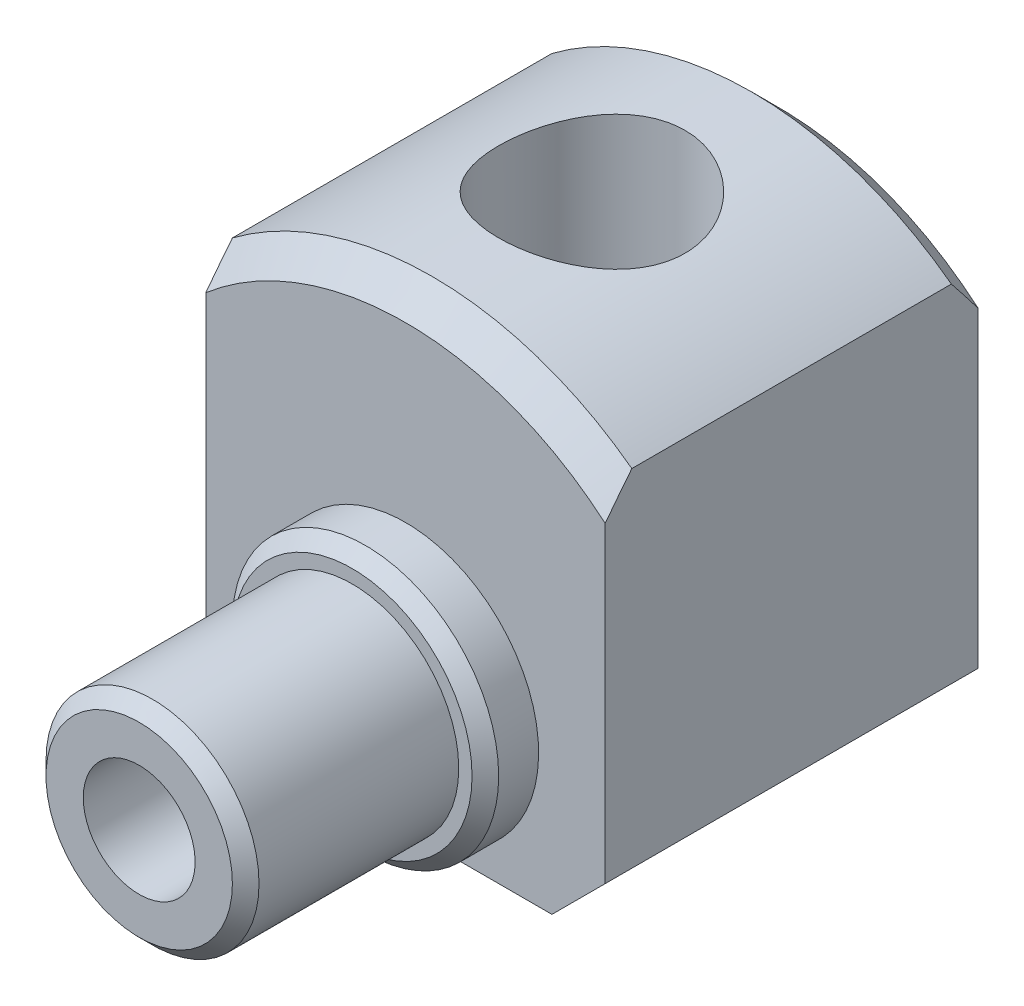
SolidWorks part; units mm, degrees
material "SUS304"
ref_plane "Front Plane" through (0, 0, 0) normal (0, 0, 1) x (1, 0, 0)
ref_plane "Top Plane" through (0, 0, 0) normal (0, 1, 0) x (1, 0, 0)
ref_plane "Right Plane" through (0, 0, 0) normal (1, 0, 0) x (0, 0, -1)
sketch "Sketch1" plane through (0, 0, 0) normal (0, 0, 1) x (1, 0, 0)
  circle A0 centre (0, 0) radius 12.5
  dimension "D1" = 25
extrude "Boss-Extrude1" add sketch "Sketch1" along normal mid plane 24
sketch "Sketch2" plane through (0, 0, 12) normal (0, 0, 1) x (1, 0, 0)
  circle A0 centre (0, 0) radius 4
  dimension "D1" = 8
extrude "Cut-Extrude1" cut sketch "Sketch2" against normal blind 10 flip side to cut
sketch "Sketch9" plane through (0, 0, -12) normal (0, 0, -1) x (-1, 0, 0)
  line L0 (0, 0) -> (0, 28.2403) construction
  line L1 (-7.5, 15) -> (7.5, 15)
  line L2 (-7.5, 15) -> (-7.5, -5)
  line L3 (-7.5, -5) -> (7.5, -5)
  line L4 (7.5, 15) -> (7.5, -5)
  dimension "D1" = 5
  dimension "D2" = 15
  dimension "D3" = 20
extrude "Cut-Extrude2" cut sketch "Sketch9" against normal through all flip side to cut
hole_wizard "M5 Tapped Hole1" positions "Sketch4" profile "Sketch3" tap size "M5" standard "GB" end condition through all
sketch "Sketch4" plane through (0, 0, -12) normal (0, 0, -1) x (-1, 0, 0)
  point P0 (0, 0)
cosmetic thread "Hole Thread1" parameters "D2"=5
sketch "Sketch3" plane through (0, 0, -12) normal (1, 0, 0) x (0, 1, 0)
  line L0 (0, 0) -> (0, 24)
  line L1 (0, 24) -> (2.1, 24)
  line L2 (2.1, 24) -> (2.1, 0)
  line L5 (2.1, 0) -> (0, 0)
  line L11 (0, -6.35) -> (0, 107.95) construction
  dimension "通孔螺纹孔钻头直径" = 4.2
  dimension "通孔螺纹孔钻头深度" = 24
sketch "Sketch8" plane through (0, 0, 2) normal (0, 0, 1) x (1, 0, 0)
  circle A0 centre (0, 0) radius 5
  circle A1 centre (0, 0) radius 4
  circle A2 centre (0, 0) radius 4 construction
  dimension "D1" = 1
extrude "Boss-Extrude2" add sketch "Sketch8" along normal blind 2
hole_wizard "M8x1.0 Tapped Hole1" positions "Sketch7" profile "Sketch6" tap size "M8x1.0" standard "GB"
sketch "Sketch7" plane through (0, 0, 0) normal (0, -1, 0) x (-1, 0, 0)
  line L0 (0, 0) -> (0, 14.4024) construction
  line L3 (7.5, 5) -> (-5.7228, 5) construction
  line L5 (7.5, -2) -> (7.5, 12) construction
  point P0 (0, 5)
sketch "Sketch6" plane through (0, 0, -5) normal (1, 0, 0) x (0, 0, -1)
  line L0 (0, 0) -> (0, 12.5)
  line L1 (0, 12.5) -> (3.5, 12.5)
  line L2 (3.5, 12.5) -> (3.5, 0)
  line L5 (3.5, 0) -> (0, 0)
  line L11 (0, -6.35) -> (0, 107.95) construction
  dimension "通孔螺纹孔钻头直径" = 7
  dimension "通孔螺纹孔钻头深度" = 12.5
cosmetic thread "Hole Thread3" parameters "D2"=8
chamfer "Chamfer1" distance 0.5 angle 45 2 edges at (4, 0, 12) (5, 0, 4)
chamfer "Chamfer2" distance 2 angle 45 2 edges at (-7.5, -5, -5) (7.5, -5, -5)
chamfer "Chamfer3" distance 1 angle 45 2 edges at (0, 12.5, 2) (0, 12.5, -12)
